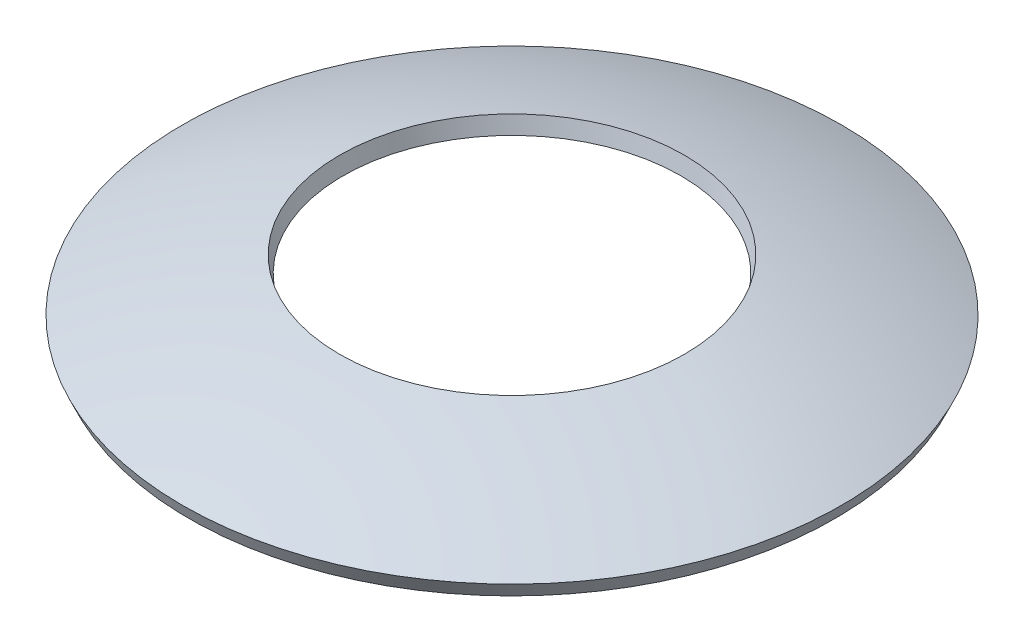
SolidWorks part; units mm, degrees
material "Brass"
ref_plane "Front" through (0, 0, 0) normal (0, 0, 1) x (1, 0, 0)
ref_plane "Top" through (0, 0, 0) normal (0, 1, 0) x (1, 0, 0)
ref_plane "Right" through (0, 0, 0) normal (1, 0, 0) x (0, 0, -1)
sketch "Sketch1" plane through (0, 0, 0) normal (1, 0, 0) x (0, 0, -1)
  line L0 (0, 0) -> (22, 0) construction
  line L1 (32.25, 46.3809) -> (32.4658, 47.3573)
  line L2 (42, 44.1843) -> (41.5876, 43.2733)
  line L3 (22, 0) -> (22, 48.4343) construction
  arc A0 (42, 44.1843) -> (32.4658, 47.3573) centre (22, 0) ccw
  arc A2 (41.5876, 43.2733) -> (32.25, 46.3809) centre (22, 0) ccw
  dimension "D2" = 95
  dimension "D3" = 97
  dimension "D1" = 22
  dimension "D4" = 10.25
  dimension "D5" = 20
revolve "Revolve1" add sketch "Sketch1" angle 360 about L3
